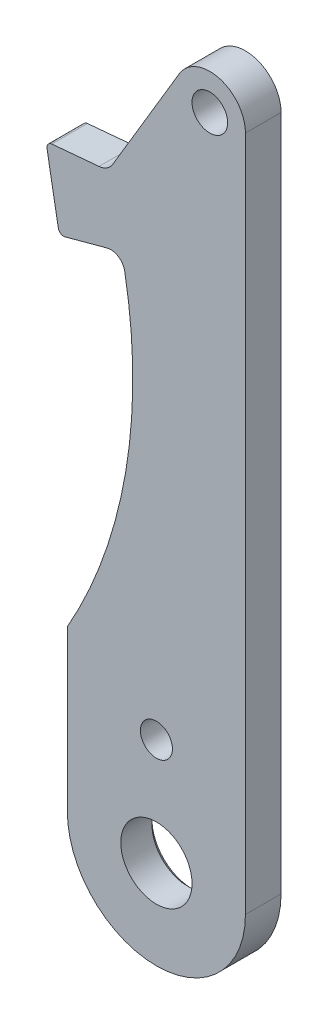
from build123d import *

# Parameters (mm, degrees)
SKETCH1_R      = 9
SKETCH1_R_2    = 10
SKETCH1_R_3    = 20
EXTRUDE1_DEPTH = 20
FILLET1_R      = 3
FILLET2_R      = 10
CHAMFER1_SIZE  = 2.5


with BuildPart() as part:
    # Sketch1 → Extrude1 (new body)
    with BuildSketch(Plane.XY):
        with BuildLine():
            Line((-54.5, 278), (-62, 320))
            Line((-62, 320), (-27.139905674, 323.126311493))
            Line((-27.139905674, 323.126311493), (12.815444518, 390.231864585))
            ThreePointArc((12.815444518, 390.231864585), (35.306076251, 399.283297302), (50, 380))
            Line((50, 380), (50, 0))
            ThreePointArc((50, 0), (0, -50), (-50, 0))
            Line((-50, 0), (-50, 90))
            ThreePointArc((-50, 90), (-17.234137889, 181.62959318), (-17.807748235, 278.939690485))
            ThreePointArc((-17.807748235, 278.939690485), (-21.406992079, 284.267795368), (-27.765067315, 285.22599012))
            Line((-27.765067315, 285.22599012), (-54.5, 278))
        make_face()
        with Locations((0, 60)):
            Circle(SKETCH1_R, mode=Mode.SUBTRACT)
        with Locations((30, 380)):
            Circle(SKETCH1_R_2, mode=Mode.SUBTRACT)
        Circle(SKETCH1_R_3, mode=Mode.SUBTRACT)
    extrude(amount=EXTRUDE1_DEPTH)

    # Fillet1
    fillet1_edges = [part.edges().sort_by_distance(p)[0] for p in [
        (-54.5, 278, 10),
        (-62, 320, 10),
    ]]
    fillet(fillet1_edges, radius=FILLET1_R)

    # Fillet2
    fillet2_edges = [part.edges().sort_by_distance(p)[0] for p in [
        (-27.139905674, 323.126311493, 10),
    ]]
    fillet(fillet2_edges, radius=FILLET2_R)

    # Chamfer1
    chamfer1_edges = [part.edges().sort_by_distance(p)[0] for p in [
        (-20, 0, 0),
    ]]
    chamfer(chamfer1_edges, length=CHAMFER1_SIZE)


solid = part.part
